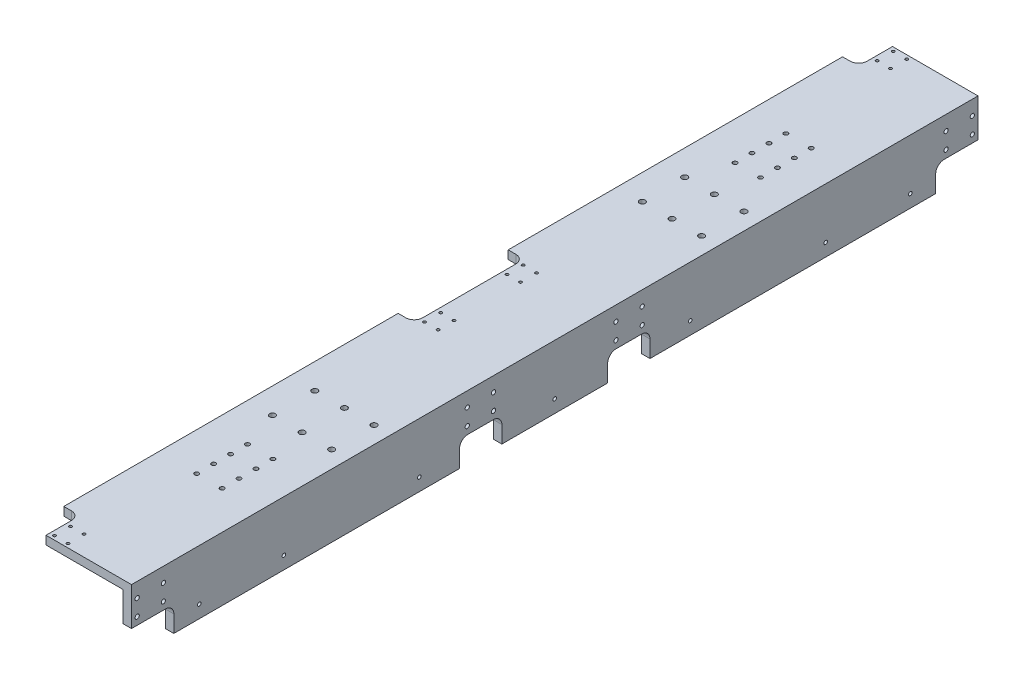
SolidWorks part; units mm, degrees
material "6061Al"
ref_plane "前视基准面" through (0, 0, 0) normal (0, 0, 1) x (1, 0, 0)
ref_plane "上视基准面" through (0, 0, 0) normal (0, 1, 0) x (1, 0, 0)
ref_plane "右视基准面" through (0, 0, 0) normal (1, 0, 0) x (0, 0, -1)
sketch "草图1" plane through (0, 0, 0) normal (0, 0, 1) x (1, 0, 0)
  line L0 (0, 0) -> (100, 0)
  line L1 (100, 0) -> (100, -90)
  line L2 (0, -10) -> (90, -10)
  line L3 (90, -10) -> (90, -90)
  line L4 (0, 0) -> (0, -10)
  line L5 (90, -90) -> (100, -90)
  dimension "D1" = 100
  dimension "D2" = 90
  dimension "D3" = 10
extrude "凸台-拉伸1" add sketch "草图1" along normal mid plane 1000
hole_wizard "M8 螺纹孔1" positions "草图6" profile "草图7" tap size "M8" standard "ISO" end condition through all
sketch "草图6" plane through (0, 0, 0) normal (0, 1, 0) x (1, 0, 0)
  line L0 (0, 0) -> (163.4287, 0) construction
  point P0 (10, -193.5)
  point P3 (10, -243.5)
  point P6 (80, -193.5)
  point P9 (80, -243.5)
  point P12 (45, -243.5)
  point P15 (45, -193.5)
  point P23 (45, 193.5)
  point P24 (45, 243.5)
  point P25 (80, 243.5)
  point P26 (80, 193.5)
  point P27 (10, 243.5)
  point P28 (10, 193.5)
sketch "草图7" plane through (10, 0, 193.5) normal (1, 0, 0) x (0, 0, 1)
  line L0 (0, 0) -> (0, 90)
  line L1 (0, 90) -> (3.4, 90)
  line L2 (3.4, 90) -> (3.4, 0)
  line L5 (3.4, 0) -> (0, 0)
  line L11 (0, -6.35) -> (0, 107.95) construction
  dimension "通孔螺纹孔钻头直径" = 6.8
  dimension "通孔螺纹孔钻头深度" = 90
cosmetic thread "孔螺蚊线37" parameters "D2"=8
cosmetic thread "孔螺蚊线38" parameters "D2"=8
cosmetic thread "孔螺蚊线39" parameters "D2"=8
cosmetic thread "孔螺蚊线40" parameters "D2"=8
cosmetic thread "孔螺蚊线41" parameters "D2"=8
cosmetic thread "孔螺蚊线42" parameters "D2"=8
cosmetic thread "孔螺蚊线43" parameters "D2"=8
cosmetic thread "孔螺蚊线44" parameters "D2"=8
cosmetic thread "孔螺蚊线45" parameters "D2"=8
cosmetic thread "孔螺蚊线46" parameters "D2"=8
cosmetic thread "孔螺蚊线47" parameters "D2"=8
cosmetic thread "孔螺蚊线48" parameters "D2"=8
other "移动面1" face at (0, -5, 0) parameters "D1"=20
other "移动面2" face at (95, -90, 0) parameters "D1"=15
chamfer "倒角1" distance 10 angle 45 4 edges at (95, -75, -500) (-20, -5, -500) (-20, -5, 500) (95, -75, 500)
sketch "草图16" plane through (0, 0, 0) normal (0, 1, 0) x (1, 0, 0)
  line L0 (-20, -490) -> (-20, 490) construction
  line L1 (-20, -460) -> (-1, -460)
  line L2 (-20, -460) -> (-20, -500)
  line L3 (-20, -500) -> (-1, -500)
  line L4 (-1, -460) -> (-1, -500)
  line L5 (100, -500) -> (-10, -500) construction
  line L7 (0, 0) -> (237.1277, 0) construction
  line L8 (-1, 460) -> (-1, 500)
  line L9 (-20, 500) -> (-1, 500)
  line L10 (-20, 460) -> (-20, 500)
  line L11 (-20, 460) -> (-1, 460)
  line L12 (-20, 65) -> (-1, 65)
  line L13 (-20, 65) -> (-20, -65)
  line L14 (-20, -65) -> (-1, -65)
  line L15 (-1, 65) -> (-1, -65)
  dimension "D1" = 19
  dimension "D2" = 40
  dimension "D3" = 130
extrude "切除-拉伸1" cut sketch "草图16" against normal through all
sketch "草图17" plane through (100, 0, 0) normal (1, 0, 0) x (0, 0, -1)
  line L0 (-490, -75) -> (490, -75) construction
  line L1 (-500, -75) -> (-450, -75)
  line L2 (-500, -75) -> (-500, -45)
  line L3 (-500, -45) -> (-450, -45)
  line L4 (-450, -75) -> (-450, -45)
  line L5 (-500, -65) -> (-500, 0) construction
  line L7 (-112.5, -75) -> (-62.5, -75)
  line L8 (-112.5, -75) -> (-112.5, -45)
  line L9 (-112.5, -45) -> (-62.5, -45)
  line L10 (-62.5, -75) -> (-62.5, -45)
  line L11 (-500, -75) -> (-112.5, -75) construction
  line L12 (0, 0) -> (0, -75) construction
  line L13 (500, -75) -> (112.5, -75) construction
  line L14 (357.8, -90) -> (357.8, 46.3525) construction
  line L15 (62.5, -75) -> (62.5, -45)
  line L16 (112.5, -45) -> (62.5, -45)
  line L17 (112.5, -75) -> (112.5, -45)
  line L18 (112.5, -75) -> (62.5, -75)
  line L19 (450, -75) -> (450, -45)
  line L20 (500, -45) -> (450, -45)
  line L21 (500, -75) -> (500, -45)
  line L22 (500, -75) -> (450, -75)
  dimension "D1" = 50
  dimension "D2" = 30
  dimension "D4" = 387.5
  dimension "D3" = 2
extrude "切除-拉伸2" cut sketch "草图17" against normal through all
hole_wizard "M6 螺纹孔1" positions "草图21" profile "草图22" tap size "M6" standard "ISO" end condition up to next
sketch "草图21" plane through (100, 0, 0) normal (1, 0, 0) x (0, 0, -1)
  line L2 (-477.8, -45.509) -> (-477.8, 21.4313) construction
  line L4 (-462.3, -36.169) -> (-462.3, -17.169) construction
  line L5 (-73.6, -45.509) -> (-42, -45.509)
  line L6 (-87.8, -45.509) -> (-87.8, 21.4313) construction
  line L7 (-72.3, -36.169) -> (-72.3, -17.169) construction
  line L8 (-462.3, -17.169) -> (-72.3, -17.169) construction
  line L9 (0, 0) -> (0, -218.4118) construction
  line L11 (462.3, -17.169) -> (72.3, -17.169) construction
  line L12 (72.3, -36.169) -> (72.3, -17.169) construction
  line L13 (87.8, -45.509) -> (87.8, 21.4313) construction
  line L14 (462.3, -36.169) -> (462.3, -17.169) construction
  line L15 (477.8, -45.509) -> (477.8, 21.4313) construction
  line L16 (73.6, -45.509) -> (42, -45.509)
  line L17 (373.6, -45.509) -> (342, -45.509)
  line L18 (-500, 0) -> (500, 0) construction
  line L20 (-500, -45) -> (-500, 0) construction
  point P0 (-493.3, -36.169)
  point P2 (-462.3, -36.169)
  point P20 (-493.3, -17.169)
  point P21 (-462.3, -17.169)
  point P27 (-103.3, -36.169)
  point P28 (-72.3, -36.169)
  point P33 (-103.3, -17.169)
  point P34 (-72.3, -17.169)
  point P55 (72.3, -17.169)
  point P56 (103.3, -17.169)
  point P57 (72.3, -36.169)
  point P58 (103.3, -36.169)
  point P59 (462.3, -17.169)
  point P60 (493.3, -17.169)
  point P61 (462.3, -36.169)
  point P62 (493.3, -36.169)
  dimension "D1" = 31
  dimension "D2" = 2
  dimension "D3" = 19
  dimension "D5" = 390
  dimension "D6" = 36.169
  dimension "D7" = 6.7
  dimension "D4" = 2
sketch "草图22" plane through (100, -36.169, 493.3) normal (0, 1, 0) x (0, 0, -1)
  line L0 (0, 0) -> (0, 10)
  line L1 (0, 10) -> (2.5, 10)
  line L2 (2.5, 10) -> (2.5, 0)
  line L5 (2.5, 0) -> (0, 0)
  line L11 (0, -6.35) -> (0, 107.95) construction
  dimension "通孔螺纹孔钻头直径" = 5
  dimension "通孔螺纹孔钻头深度" = 10
cosmetic thread "孔螺蚊线67" parameters "D2"=6
cosmetic thread "孔螺蚊线68" parameters "D2"=6
cosmetic thread "孔螺蚊线69" parameters "D2"=6
cosmetic thread "孔螺蚊线70" parameters "D2"=6
cosmetic thread "孔螺蚊线75" parameters "D2"=6
cosmetic thread "孔螺蚊线76" parameters "D2"=6
cosmetic thread "孔螺蚊线77" parameters "D2"=6
cosmetic thread "孔螺蚊线78" parameters "D2"=6
cosmetic thread "孔螺蚊线79" parameters "D2"=6
cosmetic thread "孔螺蚊线80" parameters "D2"=6
cosmetic thread "孔螺蚊线81" parameters "D2"=6
cosmetic thread "孔螺蚊线82" parameters "D2"=6
cosmetic thread "孔螺蚊线83" parameters "D2"=6
cosmetic thread "孔螺蚊线84" parameters "D2"=6
cosmetic thread "孔螺蚊线85" parameters "D2"=6
cosmetic thread "孔螺蚊线86" parameters "D2"=6
hole_wizard "M4 螺纹孔1" positions "草图23" profile "草图24" tap size "M4" standard "ISO" end condition through all
sketch "草图23" plane through (0, 0, 0) normal (0, 1, 0) x (1, 0, 0)
  line L0 (0, 0) -> (174.4572, 0) construction
  line L2 (0, 0) -> (-146.5036, 0) construction
  line L4 (100, -500) -> (-1, -500) construction
  line L5 (-20, -460) -> (-20, -65) construction
  point P0 (4.4521, -476.4)
  point P3 (20.3521, -476.4)
  point P6 (4.4521, -495.4)
  point P9 (20.3521, -495.4)
  point P12 (4.4521, -39.2)
  point P15 (4.4521, -58.2)
  point P18 (20.3521, -58.2)
  point P21 (20.3521, -39.2)
  point P30 (20.3521, 39.2)
  point P31 (20.3521, 58.2)
  point P32 (4.4521, 58.2)
  point P33 (4.4521, 39.2)
  point P51 (20.3521, 495.4)
  point P52 (4.4521, 495.4)
  point P53 (20.3521, 476.4)
  point P54 (4.4521, 476.4)
  dimension "D1" = 19
  dimension "D2" = 15.9
  dimension "D3" = 39.2
  dimension "D4" = 58.2
  dimension "D5" = 4.6
  dimension "D6" = 40.3521
  dimension "D7" = 39.2
  dimension "D8" = 58.2
sketch "草图24" plane through (4.4521, 0, 476.4) normal (1, 0, 0) x (0, 0, 1)
  line L0 (0, 0) -> (0, 75)
  line L1 (0, 75) -> (1.65, 75)
  line L2 (1.65, 75) -> (1.65, 0)
  line L5 (1.65, 0) -> (0, 0)
  line L11 (0, -6.35) -> (0, 107.95) construction
  dimension "通孔螺纹孔钻头直径" = 3.3
  dimension "通孔螺纹孔钻头深度" = 75
cosmetic thread "孔螺蚊线95" parameters "D2"=4
cosmetic thread "孔螺蚊线96" parameters "D2"=4
cosmetic thread "孔螺蚊线97" parameters "D2"=4
cosmetic thread "孔螺蚊线98" parameters "D2"=4
cosmetic thread "孔螺蚊线99" parameters "D2"=4
cosmetic thread "孔螺蚊线100" parameters "D2"=4
cosmetic thread "孔螺蚊线101" parameters "D2"=4
cosmetic thread "孔螺蚊线102" parameters "D2"=4
cosmetic thread "孔螺蚊线103" parameters "D2"=4
cosmetic thread "孔螺蚊线104" parameters "D2"=4
cosmetic thread "孔螺蚊线105" parameters "D2"=4
cosmetic thread "孔螺蚊线106" parameters "D2"=4
cosmetic thread "孔螺蚊线107" parameters "D2"=4
cosmetic thread "孔螺蚊线108" parameters "D2"=4
cosmetic thread "孔螺蚊线109" parameters "D2"=4
cosmetic thread "孔螺蚊线110" parameters "D2"=4
hole_wizard "M5 螺纹孔3" positions "草图25" profile "草图26" tap size "M5" standard "ISO" end condition through all
sketch "草图25" plane through (100, 0, 0) normal (1, 0, 0) x (0, 0, -1)
  line L0 (-420, -40.1) -> (-420, -95.9)
  line L2 (-320, -40.1) -> (-320, -95.9)
  line L4 (-160, -40.1) -> (-160, -95.9)
  line L7 (0, -95.9) -> (0, -40.1)
  line L9 (-500, 0) -> (500, 0) construction
  line L10 (160, -40.1) -> (160, -95.9)
  line L11 (320, -40.1) -> (320, -95.9)
  line L12 (420, -40.1) -> (420, -95.9)
  arc A0 (-417.1, -43) -> (-422.9, -43) centre (-420, -43) ccw construction
  arc A1 (-422.9, -93) -> (-417.1, -93) centre (-420, -93) ccw construction
  arc A2 (-317.1, -43) -> (-322.9, -43) centre (-320, -43) ccw construction
  arc A3 (-322.9, -93) -> (-317.1, -93) centre (-320, -93) ccw construction
  arc A4 (-157.1, -43) -> (-162.9, -43) centre (-160, -43) ccw construction
  arc A5 (-162.9, -93) -> (-157.1, -93) centre (-160, -93) ccw construction
  arc A6 (-2.9, -93) -> (2.9, -93) centre (0, -93) ccw construction
  arc A7 (2.9, -43) -> (-2.9, -43) centre (0, -43) ccw construction
  point P0 (-420, -60)
  point P2 (-320, -60)
  point P4 (-160, -60)
  point P6 (0, -60)
  point P58 (160, -60)
  point P59 (320, -60)
  point P60 (420, -60)
  dimension "D1" = 60
sketch "草图26" plane through (100, -60, 420) normal (0, 1, 0) x (0, 0, -1)
  line L0 (0, 0) -> (0, 120)
  line L1 (0, 120) -> (2.1, 120)
  line L2 (2.1, 120) -> (2.1, 0)
  line L5 (2.1, 0) -> (0, 0)
  line L11 (0, -6.35) -> (0, 107.95) construction
  dimension "通孔螺纹孔钻头直径" = 4.2
  dimension "通孔螺纹孔钻头深度" = 120
cosmetic thread "孔螺蚊线111" parameters "D2"=5
cosmetic thread "孔螺蚊线112" parameters "D2"=5
cosmetic thread "孔螺蚊线113" parameters "D2"=5
cosmetic thread "孔螺蚊线114" parameters "D2"=5
cosmetic thread "孔螺蚊线115" parameters "D2"=5
cosmetic thread "孔螺蚊线116" parameters "D2"=5
cosmetic thread "孔螺蚊线117" parameters "D2"=5
hole_wizard "M6 螺纹孔2" positions "草图27" profile "草图28" tap size "M6" standard "ISO" end condition through all
sketch "草图27" plane through (0, 0, 0) normal (0, 1, 0) x (1, 0, 0)
  line L1 (100, -105.8) -> (-20, -105.8) construction
  line L2 (-20, -460) -> (-20, -65) construction
  line L4 (40, -105.8) -> (40, -525.0127) construction
  line L7 (0, 0) -> (412.4967, 0) construction
  line L9 (55, -288) -> (55, -308) construction
  line L10 (55, 288) -> (55, 308) construction
  point P0 (25, -288)
  point P2 (55, -288)
  point P26 (25, -308)
  point P27 (55, -308)
  point P28 (25, -328)
  point P29 (55, -328)
  point P30 (25, -348)
  point P31 (55, -348)
  point P36 (55, 348)
  point P37 (25, 348)
  point P38 (55, 328)
  point P39 (25, 328)
  point P40 (55, 308)
  point P41 (25, 308)
  point P42 (55, 288)
  point P43 (25, 288)
  dimension "D1" = 30
  dimension "D2" = 288
  dimension "D3" = 4
  dimension "D4" = 20
sketch "草图28" plane through (25, 0, 288) normal (1, 0, 0) x (0, 0, 1)
  line L0 (0, 0) -> (0, 75)
  line L1 (0, 75) -> (2.5, 75)
  line L2 (2.5, 75) -> (2.5, 0)
  line L5 (2.5, 0) -> (0, 0)
  line L11 (0, -6.35) -> (0, 107.95) construction
  dimension "通孔螺纹孔钻头直径" = 5
  dimension "通孔螺纹孔钻头深度" = 75
cosmetic thread "孔螺蚊线118" parameters "D2"=6
cosmetic thread "孔螺蚊线119" parameters "D2"=6
cosmetic thread "孔螺蚊线120" parameters "D2"=6
cosmetic thread "孔螺蚊线121" parameters "D2"=6
cosmetic thread "孔螺蚊线122" parameters "D2"=6
cosmetic thread "孔螺蚊线123" parameters "D2"=6
cosmetic thread "孔螺蚊线124" parameters "D2"=6
cosmetic thread "孔螺蚊线125" parameters "D2"=6
cosmetic thread "孔螺蚊线126" parameters "D2"=6
cosmetic thread "孔螺蚊线127" parameters "D2"=6
cosmetic thread "孔螺蚊线128" parameters "D2"=6
cosmetic thread "孔螺蚊线129" parameters "D2"=6
cosmetic thread "孔螺蚊线130" parameters "D2"=6
cosmetic thread "孔螺蚊线131" parameters "D2"=6
cosmetic thread "孔螺蚊线132" parameters "D2"=6
cosmetic thread "孔螺蚊线133" parameters "D2"=6
fillet "圆角1" radius 10 10 edges at (95, -45, 450) (95, -45, -450) (95, -45, -112.5) (95, -45, -62.5) (95, -45, 62.5) (95, -45, 112.5) (-1, -5, 460) (-1, -5, 65) (-1, -5, -65) (-1, -5, -460)
